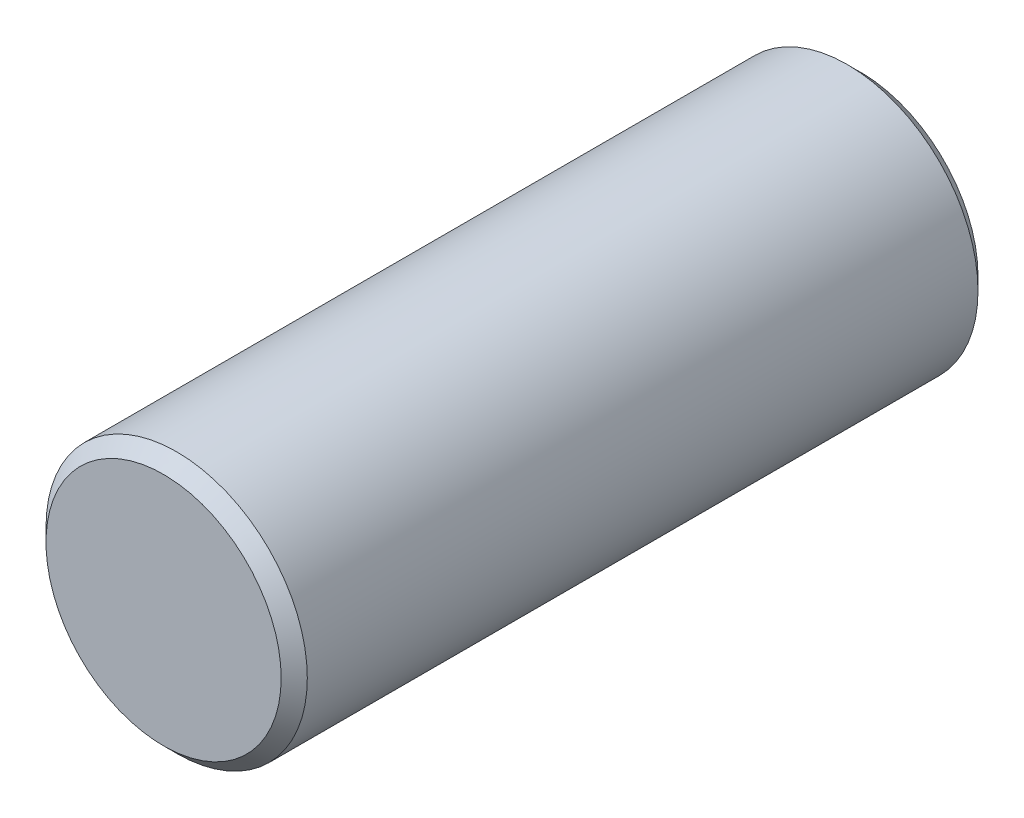
SolidWorks part; units mm, degrees
ref_plane "Front Plane" through (0, 0, 0) normal (0, 0, 1) x (1, 0, 0)
ref_plane "Top Plane" through (0, 0, 0) normal (0, 1, 0) x (1, 0, 0)
ref_plane "Right Plane" through (0, 0, 0) normal (1, 0, 0) x (0, 0, -1)
other "Configuration Table"
sketch "Sketch1" plane through (0, 0, 0) normal (0, 0, 1) x (1, 0, 0)
  circle A0 centre (0, 0) radius 3
  dimension "D1" = 6
extrude "Boss-Extrude1" add sketch "Sketch1" along normal mid plane 16
chamfer "Chamfer1" distance 0.3 angle 45 2 edges at (3, 0, -8) (3, 0, 8)
